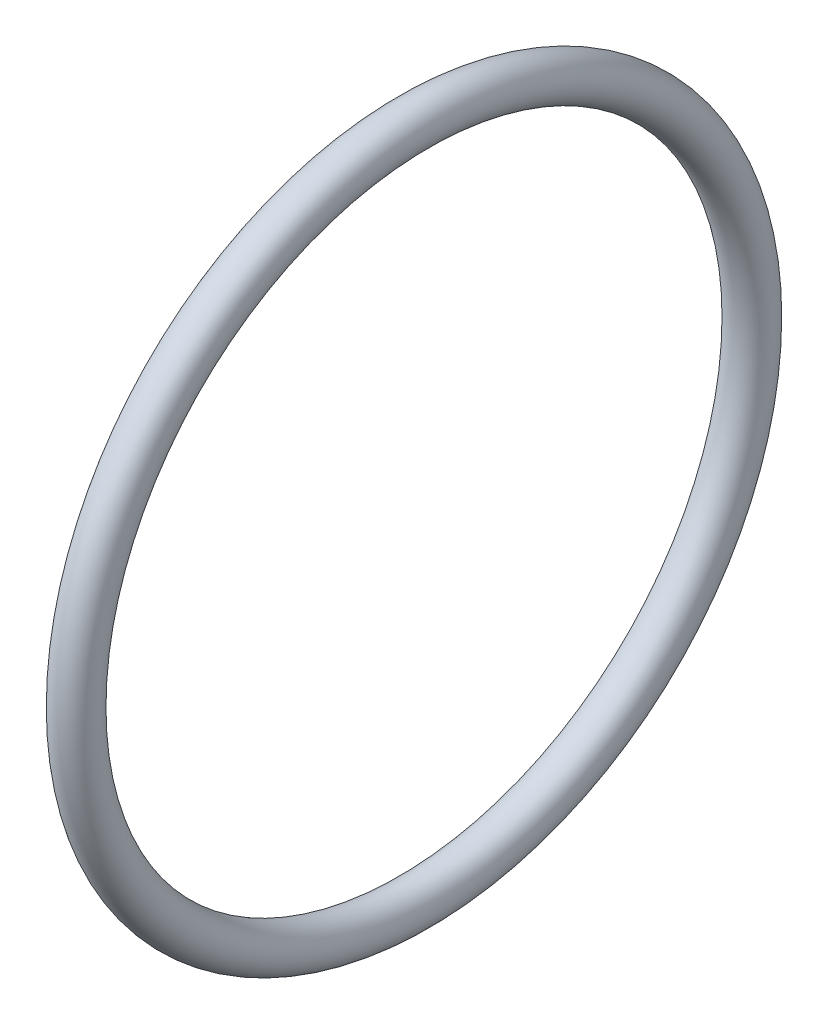
SolidWorks part; units mm, degrees
ref_plane "前视基准面" through (0, 0, 0) normal (0, 0, 1) x (1, 0, 0)
ref_plane "上视基准面" through (0, 0, 0) normal (0, 1, 0) x (1, 0, 0)
ref_plane "右视基准面" through (0, 0, 0) normal (1, 0, 0) x (0, 0, -1)
sketch "草图1" plane through (0, 0, 0) normal (0, 0, 1) x (1, 0, 0)
  line L0 (-21.9289, 0) -> (31.6751, 0) construction
  circle A0 centre (0, 40) radius 2.5
  dimension "D2" = 5
revolve "旋转1" add sketch "草图1" angle 360 about L0
sketch "草图2" plane through (0, 0, 0) normal (0, 1, 0) x (1, 0, 0)
  line L0 (-12.8648, 0) -> (21.1431, 0)
ref_plane "基准面1" through (-2.5, 0, 0) normal (1, 0, 0) x (0, 0, -1)
sketch "草图3" plane through (-2.5, 0, 0) normal (1, 0, 0) x (0, 0, -1)
  circle A0 centre (0, 0) radius 42.5
